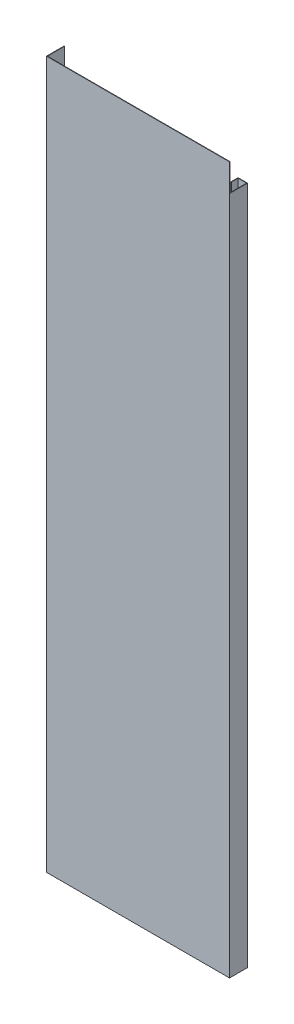
SolidWorks part; units mm, degrees
ref_plane "Front Plane" through (0, 0, 0) normal (0, 0, 1) x (1, 0, 0)
ref_plane "Top Plane" through (0, 0, 0) normal (0, 1, 0) x (1, 0, 0)
ref_plane "Right Plane" through (0, 0, 0) normal (1, 0, 0) x (0, 0, -1)
sketch "Sketch3" plane through (0, 0, 0) normal (0, 1, 0) x (1, 0, 0)
  line L0 (0, 40) -> (0, 0)
  line L1 (0, 0) -> (425, 0)
  line L2 (425, 0) -> (425, 40)
  line L3 (425, 40) -> (405, 40)
  line L4 (405, 40) -> (405, 25)
  dimension "D1" = 40
  dimension "D2" = 425
  dimension "D3" = 40
  dimension "D4" = 20
  dimension "D5" = 15
extrude "Extrude-Thin1" add sketch "Sketch3" along normal blind 1649 thin
sketch "Sketch4" plane through (0, 0, -41) normal (0, 0, -1) x (-1, 0, 0)
  line L0 (-404, 1649) -> (-404, 0) construction
  line L1 (-426, 1649) -> (-404, 1649)
  line L2 (-426, 1649) -> (-426, 1585)
  line L3 (-426, 1585) -> (-404, 1585)
  line L4 (-404, 1649) -> (-404, 1585)
  dimension "D1" = 64
extrude "Cut-Extrude1" cut sketch "Sketch4" against normal up to surface (41 mm away) up to face at (212.5, 824.5, 0)
